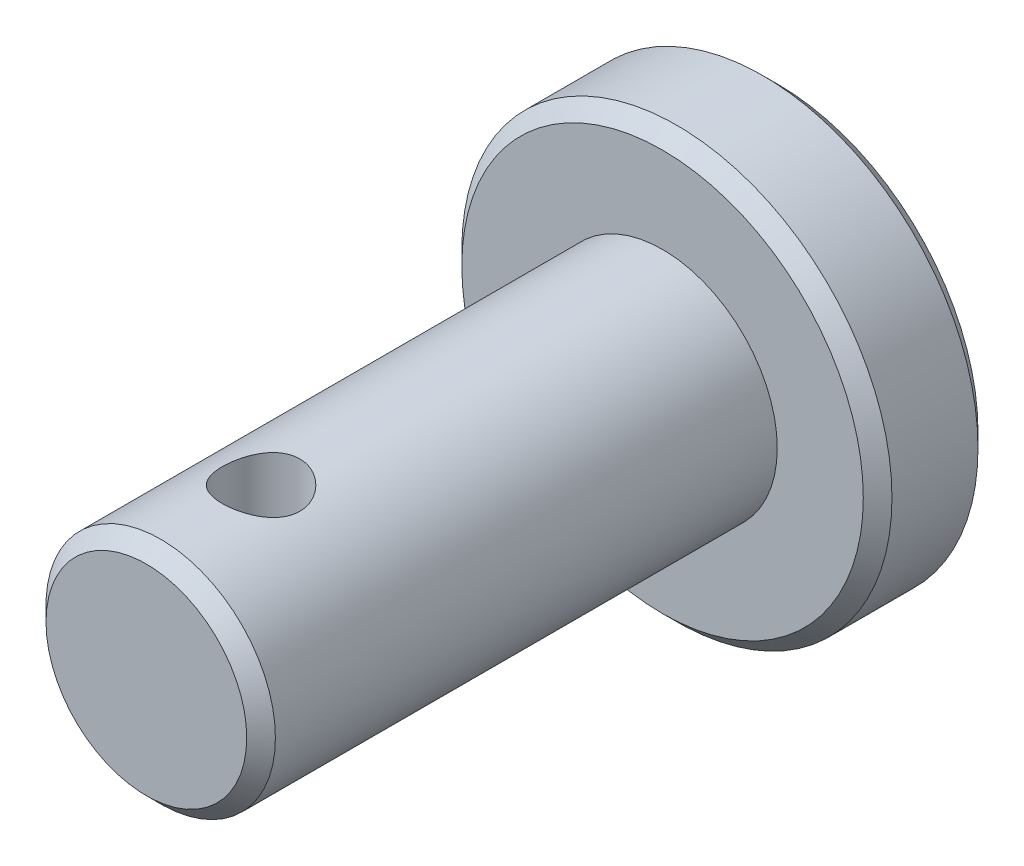
from build123d import *

# Parameters (mm, degrees)
SKETCH1_R               = 4
BOSS_EXTRUDE1_DEPTH     = 18
SKETCH2_R               = 7.5
BOSS_EXTRUDE2_DEPTH     = 4
CUT_EXTRUDE1_DEPTH      = 21.892582416
CUT_EXTRUDE1_DEPTH_BACK = 21.892582416
SKETCH3_R               = 1.35
CHAMFER1_SIZE           = 0.5


with BuildPart() as part:
    # Sketch1 → Boss-Extrude1 (new body)
    with BuildSketch(Plane.XY):
        Circle(SKETCH1_R)
    extrude(amount=BOSS_EXTRUDE1_DEPTH)

    # Sketch2 → Boss-Extrude2 (add)
    with BuildSketch(Plane(origin=(0, 0, 0), x_dir=(-1, 0, 0), z_dir=(0, 0, -1))):
        Circle(SKETCH2_R)
    extrude(amount=BOSS_EXTRUDE2_DEPTH)

    # Sketch3 → Cut-Extrude1 (cut, two sides: drawn at the far end of the back side and taken through both)
    with BuildSketch(Plane(origin=(0, 0, 0), x_dir=(1, 0, 0), z_dir=(0, 1, 0)).offset(-CUT_EXTRUDE1_DEPTH_BACK)):
        with Locations(Location((0, -14, 0), (0, 0, 270))):
            Circle(SKETCH3_R)
    extrude(amount=CUT_EXTRUDE1_DEPTH + CUT_EXTRUDE1_DEPTH_BACK, mode=Mode.SUBTRACT)

    # Chamfer1
    chamfer1_edges = [part.edges().sort_by_distance(p)[0] for p in [
        (-4, 0, 18),
        (7.5, 0, 0),
        (7.5, 0, -4),
    ]]
    chamfer(chamfer1_edges, length=CHAMFER1_SIZE)


solid = part.part
